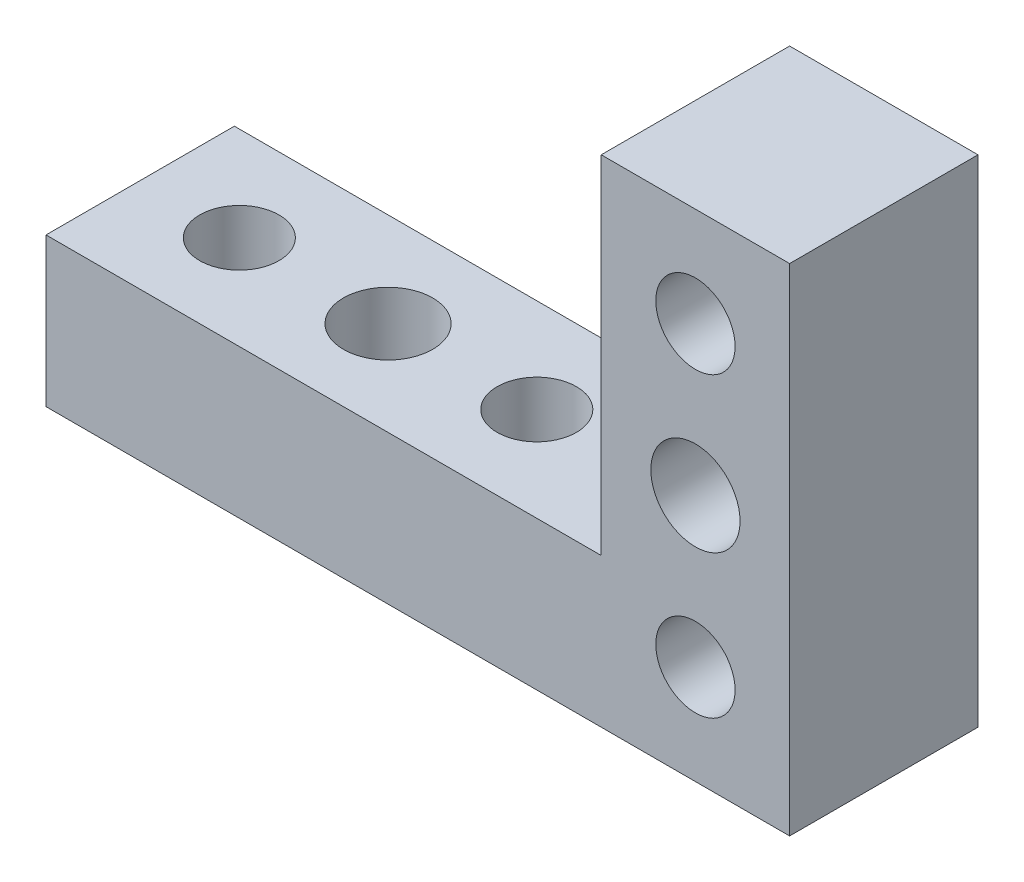
from build123d import *

# Parameters (mm, degrees)
SKETCH1_R           = 4
SKETCH1_R_2         = 4.5
BOSS_EXTRUDE1_DEPTH = 19
SKETCH2_R           = 4
SKETCH2_R_2         = 4.5
CUT_EXTRUDE1_DEPTH  = 19


with BuildPart() as part:
    # Sketch1 → Boss-Extrude1 (new body)
    with BuildSketch(Plane.XY):
        Polygon((0, 0), (75, 0), (75, 50), (56, 50), (56, 15), (0, 15), align=None)
        with Locations((65.5, 10)):
            Circle(SKETCH1_R, mode=Mode.SUBTRACT)
        with Locations((65.5, 25)):
            Circle(SKETCH1_R_2, mode=Mode.SUBTRACT)
        with Locations((65.5, 40)):
            Circle(SKETCH1_R, mode=Mode.SUBTRACT)
    extrude(amount=BOSS_EXTRUDE1_DEPTH)

    # Sketch2 → Cut-Extrude1 (cut)
    with BuildSketch(Plane(origin=(0, 15, 0), x_dir=(1, 0, 0), z_dir=(0, 1, 0))):
        with Locations(Location((10, -9.5, 0), (0, 0, 180))):
            Circle(SKETCH2_R)
        with Locations(Location((25, -9.5, 0), (0, 0, 180))):
            Circle(SKETCH2_R_2)
        with Locations(Location((40, -9.5, 0), (0, 0, 180))):
            Circle(SKETCH2_R)
    extrude(amount=-CUT_EXTRUDE1_DEPTH, mode=Mode.SUBTRACT)


solid = part.part
